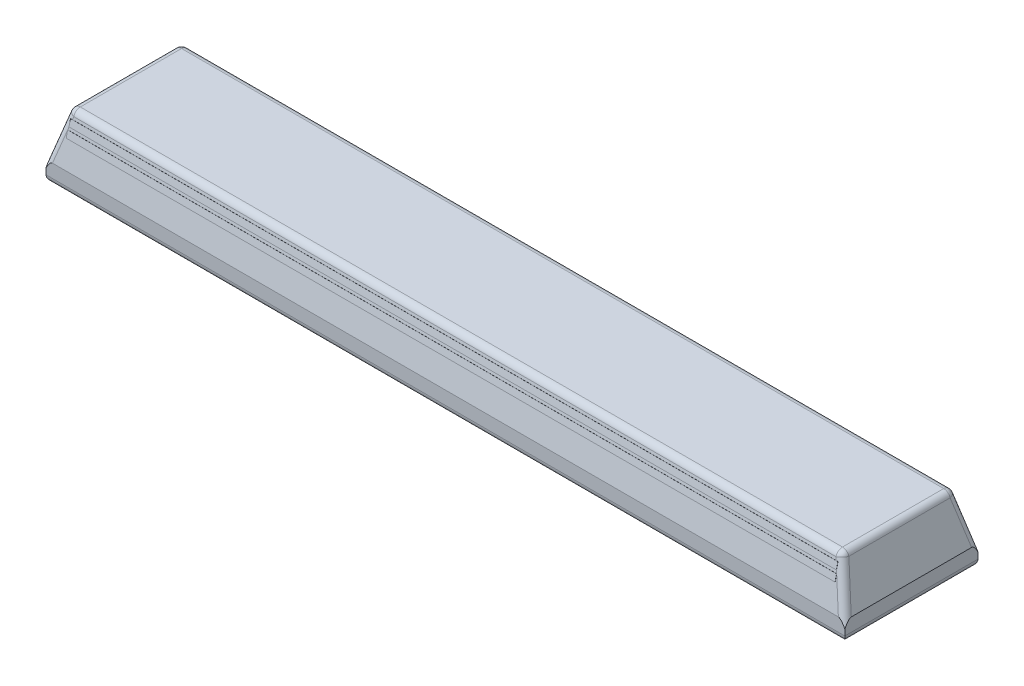
from build123d import *

# Parameters (mm, degrees)
BOSS_EXTRUDE1_DEPTH     = 500
SKETCH4_R               = 100
BOSS_EXTRUDE2_DEPTH     = 100
CUT_EXTRUDE3_DEPTH      = 6042.522986797
CUT_EXTRUDE3_DEPTH_BACK = 6042.522986797
FILLET1_R               = 50
FILLET2_R               = 20
SKETCH8_W               = 5763.564198988
SKETCH8_H               = 50
SKETCH8_W_2             = 5774.705439062
BOSS_EXTRUDE3_DEPTH     = 1


with BuildPart() as part:
    # Sketch1 → Boss-Extrude1 (new, symmetric)
    with BuildSketch(Plane.XY):
        Polygon((100, 500), (5900, 500), (6000, 150), (6000, 0), (0, 0), (0, 150), align=None)
    extrude(amount=BOSS_EXTRUDE1_DEPTH, both=True)

    # Sketch4 → Boss-Extrude2 (add)
    with BuildSketch(Plane(origin=(0, 0, 0), x_dir=(-1, 0, 0), z_dir=(0, -1, 0))):
        with Locations((-500, -250)):
            Circle(SKETCH4_R)
        with Locations((-500, 250)):
            Circle(SKETCH4_R)
        with Locations((-5500, 250)):
            Circle(SKETCH4_R)
        with Locations((-5500, -250)):
            Circle(SKETCH4_R)
        with Locations((-3000, -250)):
            Circle(SKETCH4_R)
        with Locations((-3000, 250)):
            Circle(SKETCH4_R)
    extrude(amount=BOSS_EXTRUDE2_DEPTH)

    # Sketch5 → Cut-Extrude3 (cut, two sides: drawn at the far end of the back side and taken through both)
    with BuildSketch(Plane(origin=(6000, 0, 0), x_dir=(0, 0, -1), z_dir=(1, 0, 0)).offset(-CUT_EXTRUDE3_DEPTH_BACK)):
        Polygon((-420, 500), (-500, 150), (-500, 500), align=None)
        Polygon((500, 500), (500, 150), (420, 500), align=None)
    extrude(amount=CUT_EXTRUDE3_DEPTH + CUT_EXTRUDE3_DEPTH_BACK, mode=Mode.SUBTRACT)

    # Fillet1
    fillet1_edges = [part.edges().sort_by_distance(p)[0] for p in [
        (5900, 500, 0),
        (100, 500, 0),
        (6000, 0, 0),
        (3000, 0, -500),
        (3000, 0, 500),
        (0, 0, 0),
        (5950, 325, -460),
        (5950, 325, 460),
        (50, 325, 460),
        (50, 325, -460),
        (3000, 500, -420),
        (3000, 500, 420),
    ]]
    fillet(fillet1_edges, radius=FILLET1_R)

    # Fillet2
    fillet2_edges = [part.edges().sort_by_distance(p)[0] for p in [
        (600, -100, 250),
        (600, -100, -250),
        (5600, -100, -250),
        (5600, -100, 250),
        (3100, -100, 250),
        (3100, -100, -250),
    ]]
    fillet(fillet2_edges, radius=FILLET2_R)

    # Sketch8 → Boss-Extrude3 (add)
    with BuildSketch(Plane(origin=(0, 116.058960434, 507.757951901), x_dir=(1, 0, 0), z_dir=(0, 0.22282480150214157, 0.9748585065718672))):
        with Locations((3000, 308.981913595)):
            Rectangle(SKETCH8_W, SKETCH8_H)
        with Locations((3000, 238.981913595)):
            Rectangle(SKETCH8_W_2, SKETCH8_H)
    extrude(amount=BOSS_EXTRUDE3_DEPTH)


solid = part.part
